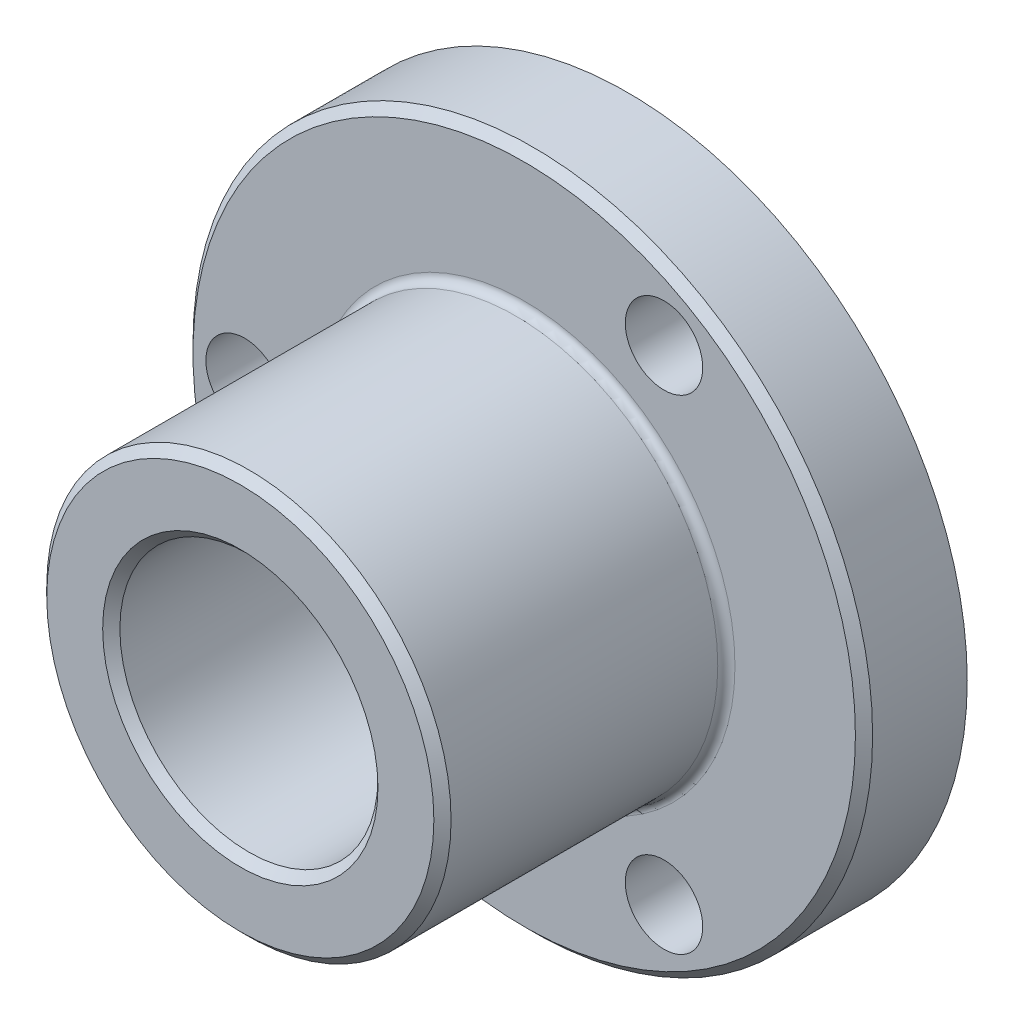
SolidWorks part; units mm, degrees
material "1023 碳钢板 (SS)"
ref_plane "Front Plane" through (0, 0, 0) normal (0, 0, 1) x (1, 0, 0)
ref_plane "Top Plane" through (0, 0, 0) normal (0, 1, 0) x (1, 0, 0)
ref_plane "Right Plane" through (0, 0, 0) normal (1, 0, 0) x (0, 0, -1)
sketch "Sketch1" plane through (0, 0, 0) normal (0, 0, 1) x (1, 0, 0)
  circle A0 centre (0, 0) radius 39.5
  dimension "D1" = 79
extrude "Boss-Extrude1" add sketch "Sketch1" along normal blind 12
sketch "Sketch2" plane through (0, 0, 12) normal (0, 0, 1) x (1, 0, 0)
  circle A0 centre (0, 0) radius 23.5
  dimension "D1" = 47
extrude "Boss-Extrude2" add sketch "Sketch2" along normal blind 33
sketch "Sketch3" plane through (0, 0, 45) normal (0, 0, 1) x (1, 0, 0)
  circle A0 centre (0, 0) radius 15
  dimension "D1" = 30
extrude "Cut-Extrude1" cut sketch "Sketch3" against normal blind 35
sketch "Sketch4" plane through (0, 0, 10) normal (0, 0, 1) x (1, 0, 0)
  circle A0 centre (0, 0) radius 5.5
  dimension "D1" = 11
extrude "Cut-Extrude2" cut sketch "Sketch4" against normal blind 3
sketch "Sketch5" plane through (0, 0, 7) normal (0, 0, 1) x (1, 0, 0)
  circle A1 centre (0, 0) radius 5.5
  circle A2 centre (0, 0) radius 5.5
  dimension "D1" = 0
extrude "Cut-Extrude3" cut sketch "Sketch5" against normal blind 7 draft 45 draft outward yes
chamfer "Chamfer1" distance 1 angle 45 3 edges at (39.5, 0, 12) (23.5, 0, 45) (15, 0, 45)
sketch "Sketch6" plane through (0, 0, 0) normal (0, 0, -1) x (-1, 0, 0)
  line L0 (0, 0) -> (32.5, 0) construction
  line L1 (0, 0) -> (-16.25, -28.1458) construction
  line L2 (0, 0) -> (-16.25, 28.1458) construction
  circle A0 centre (0, 0) radius 32.5 construction
  circle A1 centre (32.5, 0) radius 4.5
  circle A2 centre (-16.25, -28.1458) radius 4.5
  circle A3 centre (-16.25, 28.1458) radius 4.5
  dimension "D1" = 65
  dimension "D4" = 9
  dimension "D2" = 120
  dimension "D3" = 120
extrude "Cut-Extrude4" cut sketch "Sketch6" against normal blind 21
fillet "Fillet1" radius 1 2 edges at (15, 0, 10) (23.5, 0, 12)
